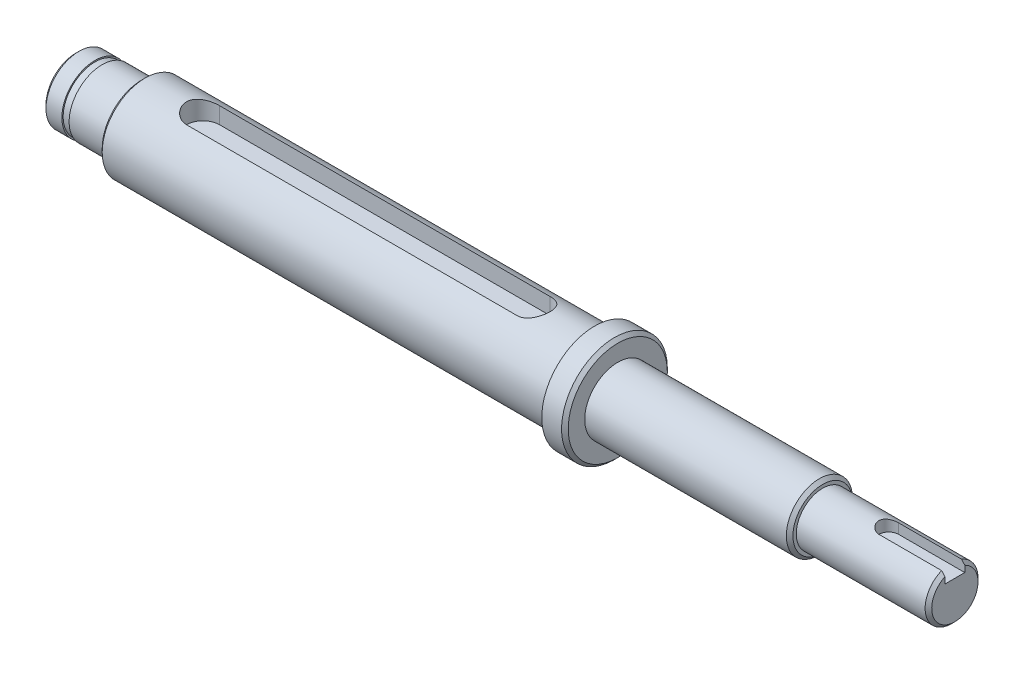
from build123d import *

# Parameters (mm, degrees)
CUT_EXTRUDE_START   = 4
CUT_EXTRUDE_1_DEPTH = 1.8
CHAMFER_1_SIZE      = 0.5
CUT_EXTRUDE_3_DEPTH = 3


with BuildPart() as part:
    # 草图1 → 旋转1 (revolve)
    with BuildSketch(Plane.XY, mode=Mode.PRIVATE) as revolve_1_sk:
        Polygon((-133, 5), (-130.1, 5), (-130.1, 4.8), (-129, 4.8), (-129, 5), (-123, 5), (-123, 6.5), (-54.5, 6.5), (-54.5, 8), (-51, 8), (-51, 5), (-20, 5), (-20, 4), (0, 4), (0, 0), (-133, 0), align=None)
    revolve(revolve_1_sk.sketch.rotate(Axis((0, 0, 0), (-1, 0, 0)), 90), axis=Axis((0, 0, 0), (-1, 0, 0)))

    # 草图2 → 切除-拉伸1 (cut)
    with BuildSketch(Plane(origin=(0, 0, 0), x_dir=(1, 0, 0), z_dir=(0, 1, 0)).offset(CUT_EXTRUDE_START)):
        with BuildLine():
            Line((-10, 1.5), (0, 1.5))
            ThreePointArc((0, 1.5), (1.5, 0), (0, -1.5))
            Line((0, -1.5), (-10, -1.5))
            ThreePointArc((-10, -1.5), (-11.5, 0), (-10, 1.5))
        make_face()
    extrude(amount=-CUT_EXTRUDE_1_DEPTH, mode=Mode.SUBTRACT)

    # 倒角1
    chamfer_1_edges = [part.edges().sort_by_distance(p)[0] for p in [
        (-20, 0, 5),
        (-51, 0, 8),
        (-123, 0, 6.5),
        (-133, 0, 5),
        (0, -3.31662479, 2.236067977),
    ]]
    chamfer(chamfer_1_edges, length=CHAMFER_1_SIZE)

    # 草图4 → 切除-拉伸3 (cut)
    with BuildSketch(Plane(origin=(0, 6.5, 0), x_dir=(1, 0, 0), z_dir=(0, 1, 0))):
        with BuildLine():
            Line((-113.75, 2.5), (-63.75, 2.5))
            ThreePointArc((-63.75, 2.5), (-61.25, 0), (-63.75, -2.5))
            Line((-63.75, -2.5), (-113.75, -2.5))
            ThreePointArc((-113.75, -2.5), (-116.25, 0), (-113.75, 2.5))
        make_face()
    extrude(amount=-CUT_EXTRUDE_3_DEPTH, mode=Mode.SUBTRACT)


solid = part.part
